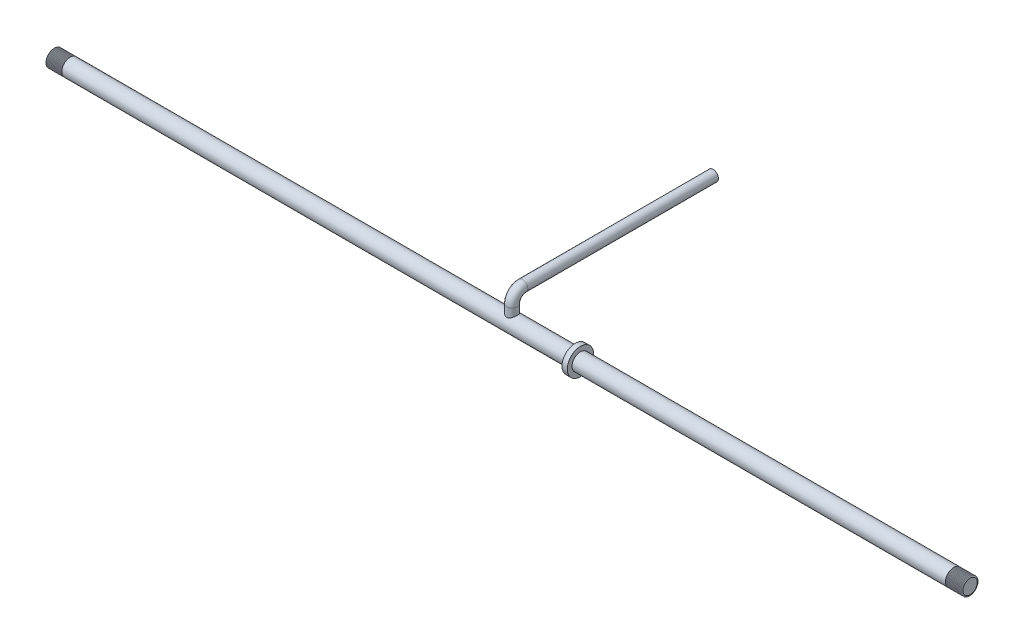
from build123d import *

# Parameters (mm, degrees)
SKETCH_3_R             = 5
SKETCH_4_R             = 8
EXTRUDE_2_DEPTH        = 435
PATTERN_LINEAR_1_COUNT = 16
PATTERN_LINEAR_1_PITCH = 1
SKETCH_8_R             = 12.5
EXTRUDE_3_DEPTH        = 5


with BuildPart() as part:
    # 扫描1: sweep along a path in 草图2
    with BuildLine(Plane(origin=(0, 0, 0), x_dir=(0, 0, -1), z_dir=(1, 0, 0))) as sweep_1_path:
        Line((0, 0), (0, 15))
        ThreePointArc((0, 15), (2.928932188, 22.071067812), (10, 25))
        Line((10, 25), (191, 25))
    # 草图3 → 扫描1 (sweep)
    with BuildSketch(Plane(origin=(0, 0, 0), x_dir=(1, 0, 0), z_dir=(0, 1, 0))):
        Circle(SKETCH_3_R)
    sweep(path=sweep_1_path.line)


with BuildPart() as body_2:
    # 草图4 → 凸台-拉伸2 (new, symmetric)
    with BuildSketch(Plane(origin=(0, 0, 0), x_dir=(0, 0, -1), z_dir=(1, 0, 0))):
        with Locations(Location((0, 0, 0), (0, 0, 180))):
            Circle(SKETCH_4_R)
    extrude(amount=EXTRUDE_2_DEPTH, both=True)

    # 草图7 → 切除-旋转1 (revolve, cut)
    with BuildSketch(Plane(origin=(0, 0, 0), x_dir=(1, 0, 0), z_dir=(0, 1, 0)), mode=Mode.PRIVATE) as cut_revolve_1_sk:
        Polygon((420, 8), (420.5, 8), (420, 6.8), (419.5, 8), align=None)
    cut_revolve_1 = revolve(cut_revolve_1_sk.sketch.rotate(Axis((442.161138775, 0, 0), (-1, 0, 0)), 180), axis=Axis((442.161138775, 0, 0), (-1, 0, 0)), mode=Mode.SUBTRACT)

    # 阵列(线性)1: 切除-旋转1 ×16
    with Locations(*[(i * PATTERN_LINEAR_1_PITCH, 0, 0) for i in range(1, PATTERN_LINEAR_1_COUNT)]):
        add(cut_revolve_1, mode=Mode.SUBTRACT)

    # 镜向2: 切除-旋转1 across plane
    add(cut_revolve_1.mirror(Plane(origin=(0, 0, 0), x_dir=(0, 0, 1), z_dir=(1, 0, 0))), mode=Mode.SUBTRACT)

    # 镜向2 copy 1 sketch → 镜向2 copy 1 (revolve, cut)
    with BuildSketch(Plane(origin=(-1, 0, 0), x_dir=(-1, 0, 0), z_dir=(0, 1, 0))):
        Polygon((420, -8), (420.5, -8), (420, -6.8), (419.5, -8), align=None)
    revolve(axis=Axis((-443.161138775, 0, 0), (-1, 0, 0)), mode=Mode.SUBTRACT)

    # 镜向2 copy 2 sketch → 镜向2 copy 2 (revolve, cut)
    with BuildSketch(Plane(origin=(-2, 0, 0), x_dir=(-1, 0, 0), z_dir=(0, 1, 0))):
        Polygon((420, -8), (420.5, -8), (420, -6.8), (419.5, -8), align=None)
    revolve(axis=Axis((-444.161138775, 0, 0), (-1, 0, 0)), mode=Mode.SUBTRACT)

    # 镜向2 copy 3 sketch → 镜向2 copy 3 (revolve, cut)
    with BuildSketch(Plane(origin=(-3, 0, 0), x_dir=(-1, 0, 0), z_dir=(0, 1, 0))):
        Polygon((420, -8), (420.5, -8), (420, -6.8), (419.5, -8), align=None)
    revolve(axis=Axis((-445.161138775, 0, 0), (-1, 0, 0)), mode=Mode.SUBTRACT)

    # 镜向2 copy 4 sketch → 镜向2 copy 4 (revolve, cut)
    with BuildSketch(Plane(origin=(-4, 0, 0), x_dir=(-1, 0, 0), z_dir=(0, 1, 0))):
        Polygon((420, -8), (420.5, -8), (420, -6.8), (419.5, -8), align=None)
    revolve(axis=Axis((-446.161138775, 0, 0), (-1, 0, 0)), mode=Mode.SUBTRACT)

    # 镜向2 copy 5 sketch → 镜向2 copy 5 (revolve, cut)
    with BuildSketch(Plane(origin=(-5, 0, 0), x_dir=(-1, 0, 0), z_dir=(0, 1, 0))):
        Polygon((420, -8), (420.5, -8), (420, -6.8), (419.5, -8), align=None)
    revolve(axis=Axis((-447.161138775, 0, 0), (-1, 0, 0)), mode=Mode.SUBTRACT)

    # 镜向2 copy 6 sketch → 镜向2 copy 6 (revolve, cut)
    with BuildSketch(Plane(origin=(-6, 0, 0), x_dir=(-1, 0, 0), z_dir=(0, 1, 0))):
        Polygon((420, -8), (420.5, -8), (420, -6.8), (419.5, -8), align=None)
    revolve(axis=Axis((-448.161138775, 0, 0), (-1, 0, 0)), mode=Mode.SUBTRACT)

    # 镜向2 copy 7 sketch → 镜向2 copy 7 (revolve, cut)
    with BuildSketch(Plane(origin=(-7, 0, 0), x_dir=(-1, 0, 0), z_dir=(0, 1, 0))):
        Polygon((420, -8), (420.5, -8), (420, -6.8), (419.5, -8), align=None)
    revolve(axis=Axis((-449.161138775, 0, 0), (-1, 0, 0)), mode=Mode.SUBTRACT)

    # 镜向2 copy 8 sketch → 镜向2 copy 8 (revolve, cut)
    with BuildSketch(Plane(origin=(-8, 0, 0), x_dir=(-1, 0, 0), z_dir=(0, 1, 0))):
        Polygon((420, -8), (420.5, -8), (420, -6.8), (419.5, -8), align=None)
    revolve(axis=Axis((-450.161138775, 0, 0), (-1, 0, 0)), mode=Mode.SUBTRACT)

    # 镜向2 copy 9 sketch → 镜向2 copy 9 (revolve, cut)
    with BuildSketch(Plane(origin=(-9, 0, 0), x_dir=(-1, 0, 0), z_dir=(0, 1, 0))):
        Polygon((420, -8), (420.5, -8), (420, -6.8), (419.5, -8), align=None)
    revolve(axis=Axis((-451.161138775, 0, 0), (-1, 0, 0)), mode=Mode.SUBTRACT)

    # 镜向2 copy 10 sketch → 镜向2 copy 10 (revolve, cut)
    with BuildSketch(Plane(origin=(-10, 0, 0), x_dir=(-1, 0, 0), z_dir=(0, 1, 0))):
        Polygon((420, -8), (420.5, -8), (420, -6.8), (419.5, -8), align=None)
    revolve(axis=Axis((-452.161138775, 0, 0), (-1, 0, 0)), mode=Mode.SUBTRACT)

    # 镜向2 copy 11 sketch → 镜向2 copy 11 (revolve, cut)
    with BuildSketch(Plane(origin=(-11, 0, 0), x_dir=(-1, 0, 0), z_dir=(0, 1, 0))):
        Polygon((420, -8), (420.5, -8), (420, -6.8), (419.5, -8), align=None)
    revolve(axis=Axis((-453.161138775, 0, 0), (-1, 0, 0)), mode=Mode.SUBTRACT)

    # 镜向2 copy 12 sketch → 镜向2 copy 12 (revolve, cut)
    with BuildSketch(Plane(origin=(-12, 0, 0), x_dir=(-1, 0, 0), z_dir=(0, 1, 0))):
        Polygon((420, -8), (420.5, -8), (420, -6.8), (419.5, -8), align=None)
    revolve(axis=Axis((-454.161138775, 0, 0), (-1, 0, 0)), mode=Mode.SUBTRACT)

    # 镜向2 copy 13 sketch → 镜向2 copy 13 (revolve, cut)
    with BuildSketch(Plane(origin=(-13, 0, 0), x_dir=(-1, 0, 0), z_dir=(0, 1, 0))):
        Polygon((420, -8), (420.5, -8), (420, -6.8), (419.5, -8), align=None)
    revolve(axis=Axis((-455.161138775, 0, 0), (-1, 0, 0)), mode=Mode.SUBTRACT)

    # 镜向2 copy 14 sketch → 镜向2 copy 14 (revolve, cut)
    with BuildSketch(Plane(origin=(-14, 0, 0), x_dir=(-1, 0, 0), z_dir=(0, 1, 0))):
        Polygon((420, -8), (420.5, -8), (420, -6.8), (419.5, -8), align=None)
    revolve(axis=Axis((-456.161138775, 0, 0), (-1, 0, 0)), mode=Mode.SUBTRACT)

    # 镜向2 copy 15 sketch → 镜向2 copy 15 (revolve, cut)
    with BuildSketch(Plane(origin=(-15, 0, 0), x_dir=(-1, 0, 0), z_dir=(0, 1, 0))):
        Polygon((420, -8), (420.5, -8), (420, -6.8), (419.5, -8), align=None)
    revolve(axis=Axis((-457.161138775, 0, 0), (-1, 0, 0)), mode=Mode.SUBTRACT)

    # 草图8 → 凸台-拉伸3 (add)
    with BuildSketch(Plane(origin=(60, 0, 0), x_dir=(0, 0, -1), z_dir=(1, 0, 0))):
        Circle(SKETCH_8_R)
    extrude(amount=EXTRUDE_3_DEPTH)


solid = Compound([part.part, body_2.part])
